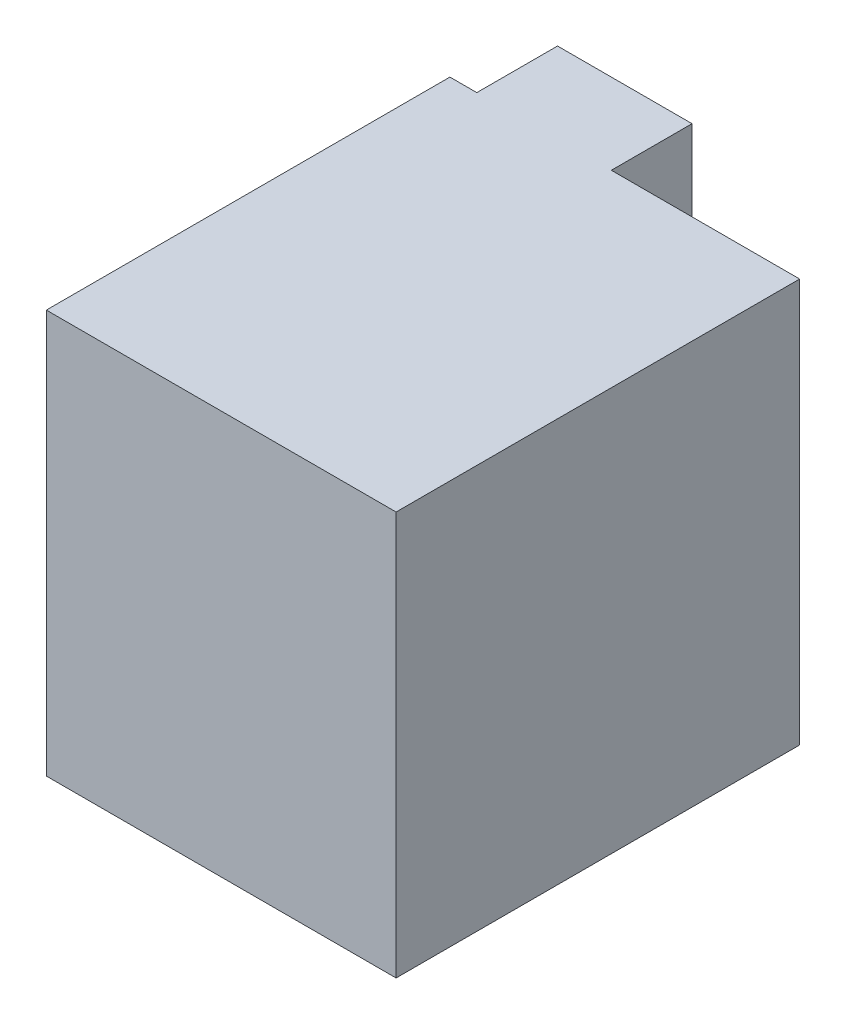
SolidWorks part; units mm, degrees
ref_plane "前视基准面" through (0, 0, 0) normal (0, 0, 1) x (1, 0, 0)
ref_plane "上视基准面" through (0, 0, 0) normal (0, 1, 0) x (1, 0, 0)
ref_plane "右视基准面" through (0, 0, 0) normal (1, 0, 0) x (0, 0, -1)
sketch "草图1" plane through (0, 0, 0) normal (0, 1, 0) x (1, 0, 0)
  line L0 (0, 0) -> (130, 0)
  line L1 (130, 0) -> (130, 150)
  line L2 (130, 150) -> (60, 150)
  line L3 (60, 150) -> (60, 180)
  line L4 (60, 180) -> (10, 180)
  line L5 (10, 180) -> (10, 150)
  line L6 (10, 150) -> (0, 150)
  line L7 (0, 150) -> (0, 0)
  dimension "D1" = 130
  dimension "D2" = 150
  dimension "D3" = 50
  dimension "D4" = 70
  dimension "D5" = 30
extrude "凸台-拉伸1" add sketch "草图1" along normal blind 150
